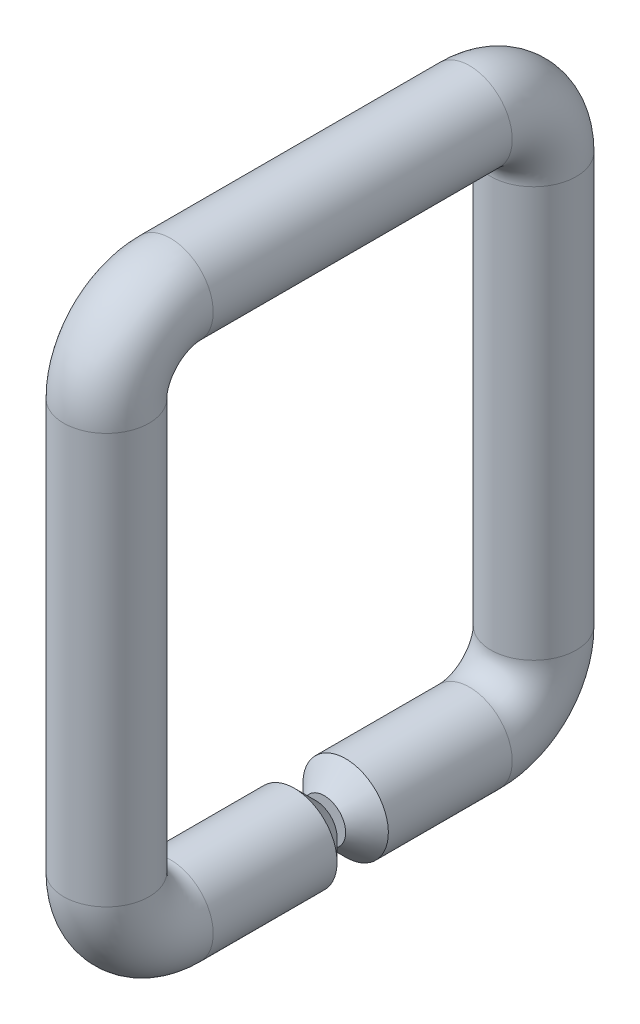
from build123d import *

# Parameters (mm, degrees)
SKETCH2_R     = 10
CHAMFER1_SIZE = 5


with BuildPart() as part:
    # Sweep1: sweep along a path in Sketch4
    with BuildLine(Plane(origin=(0, 0, 0), x_dir=(0, 0, -1), z_dir=(1, 0, 0))) as sweep1_path:
        Line((0, 0), (-34, 0))
        ThreePointArc((-34, 0), (-44.606601718, 4.393398282), (-49, 15))
        Line((-49, 15), (-49, 111))
        ThreePointArc((-49, 111), (-44.606601718, 121.606601718), (-34, 126))
        Line((-34, 126), (36, 126))
        ThreePointArc((36, 126), (46.606601718, 121.606601718), (51, 111))
        Line((51, 111), (51, 15))
        ThreePointArc((51, 15), (46.606601718, 4.393398282), (36, 0))
        Line((36, 0), (2, 0))
    # Sketch2 → Sweep1 (sweep)
    with BuildSketch(Plane.XY):
        Circle(SKETCH2_R)
    sweep(path=sweep1_path.line)

    # Chamfer1
    chamfer1_edges = [part.edges().sort_by_distance(p)[0] for p in [
        (-10, 0, -2),
        (-10, 0, 0),
    ]]
    chamfer(chamfer1_edges, length=CHAMFER1_SIZE)


solid = part.part
